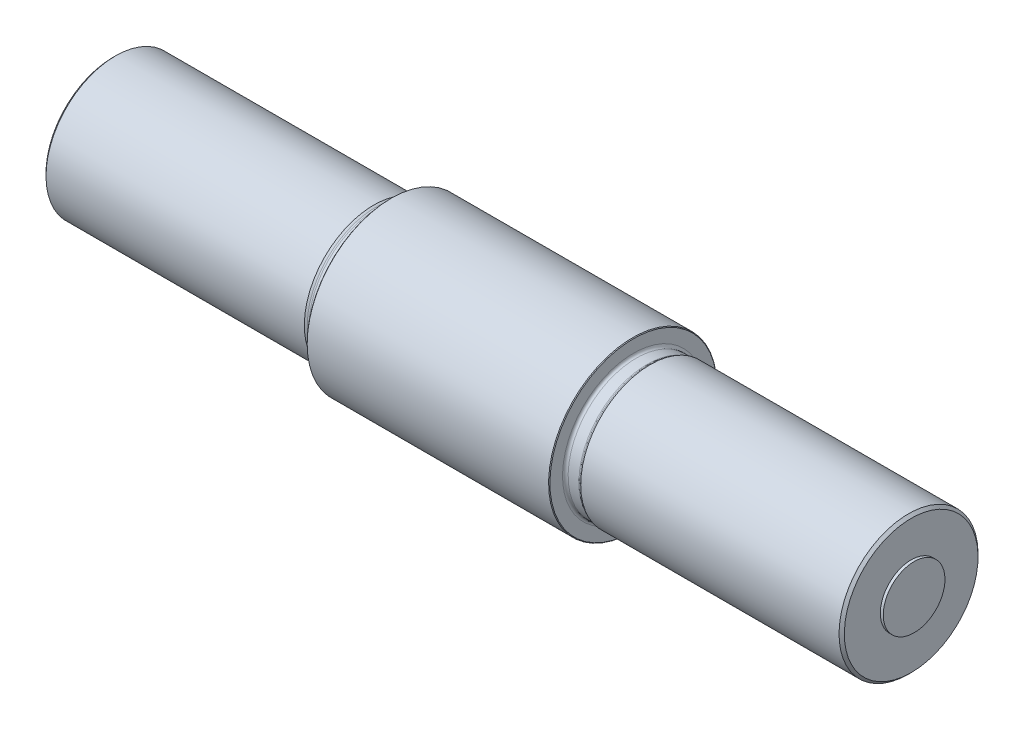
from build123d import *

# Parameters (mm, degrees)
CHAMFER1_SIZE      = 3
CHAMFER2_SIZE      = 0.762
FILLET1_R          = 3.175
SKETCH2_R          = 11.3157
CUT_EXTRUDE1_DEPTH = 28.702


with BuildPart() as part:
    # Sketch1 → Revolve1 (revolve)
    with BuildSketch(Plane.XY, mode=Mode.PRIVATE) as revolve1_sk:
        Polygon((137.3251, 95.2119), (-137.3251, 95.2119), (-137.3251, 77.0001), (-153.548479685, 77.0001), (-156.3751, 78.63205), (-451.6501, 78.63205), (-451.6501, 34.925), (-454.9521, 34.925), (-454.9521, 0), (454.9521, 0), (454.9521, 34.925), (451.6501, 34.925), (451.6501, 78.63205), (156.3751, 78.63205), (153.548479685, 77.0001), (137.3251, 77.0001), align=None)
    revolve(revolve1_sk.sketch.rotate(Axis((-454.9521, 0, 0), (1, 0, 0)), 180), axis=Axis((-454.9521, 0, 0), (1, 0, 0)))

    # Chamfer1
    chamfer1_edges = [part.edges().sort_by_distance(p)[0] for p in [
        (-451.6501, 78.63205, 0),
        (451.6501, 78.63205, 0),
    ]]
    chamfer(chamfer1_edges, length=CHAMFER1_SIZE)

    # Chamfer2
    chamfer2_edges = [part.edges().sort_by_distance(p)[0] for p in [
        (137.3251, 95.2119, 0),
        (-137.3251, 95.2119, 0),
    ]]
    chamfer(chamfer2_edges, length=CHAMFER2_SIZE)

    # Fillet1
    fillet1_edges = [part.edges().sort_by_distance(p)[0] for p in [
        (-137.3251, 77.0001, 0),
        (-153.548479685, 77.0001, 0),
        (153.548479685, 77.0001, 0),
        (137.3251, 77.0001, 0),
    ]]
    fillet(fillet1_edges, radius=FILLET1_R)

    # Sketch2 → Cut-Extrude1 (cut)
    with BuildSketch(Plane(origin=(0, 0, -95.2119), x_dir=(0, -1, 0), z_dir=(0, 0, -1))):
        with Locations(Location((0, 0, 0), (0, 0, 180))):
            Circle(SKETCH2_R)
    extrude(amount=-CUT_EXTRUDE1_DEPTH, mode=Mode.SUBTRACT)


solid = part.part
